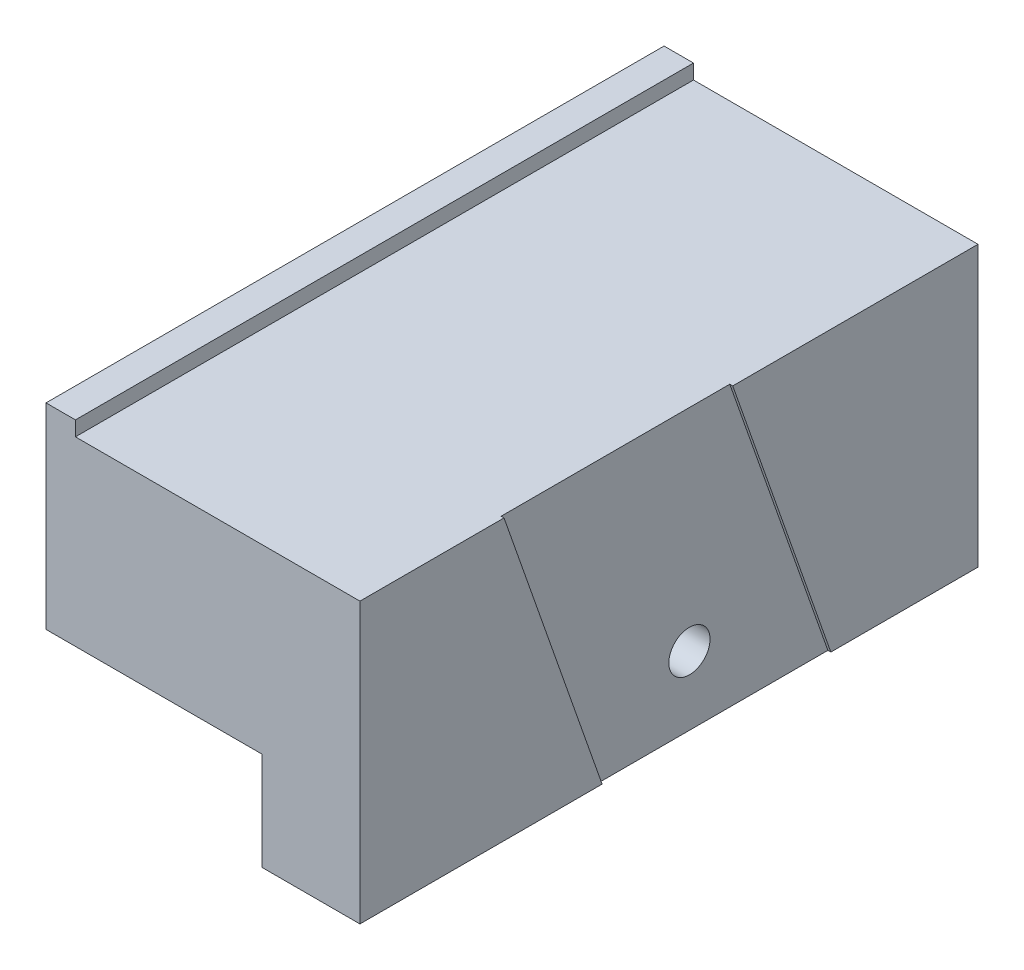
SolidWorks part; units mm, degrees
ref_plane "前视基准面" through (0, 0, 0) normal (0, 0, 1) x (1, 0, 0)
ref_plane "上视基准面" through (0, 0, 0) normal (0, 1, 0) x (1, 0, 0)
ref_plane "右视基准面" through (0, 0, 0) normal (1, 0, 0) x (0, 0, -1)
sketch "草图1" plane through (0, 0, 0) normal (0, 0, 1) x (1, 0, 0)
  line L0 (0, 0) -> (32, 0)
  line L1 (32, 0) -> (32, -30)
  line L2 (32, -30) -> (22, -30)
  line L3 (22, -30) -> (22, -20)
  line L4 (22, -20) -> (0, -20)
  line L5 (0, -20) -> (0, 0)
  dimension "D1" = 20
  dimension "D2" = 10
  dimension "D3" = 32
  dimension "D4" = 10
extrude "凸台-拉伸1" add sketch "草图1" along normal mid plane 63
sketch "草图2" plane through (0, 0, 0) normal (0, 1, 0) x (1, 0, 0)
  line L0 (32, -31.5) -> (0, -31.5) construction
  line L1 (32, 31.5) -> (3, 31.5)
  line L2 (32, 31.5) -> (32, -31.5)
  line L3 (32, -31.5) -> (3, -31.5)
  line L4 (3, 31.5) -> (3, -31.5)
  line L5 (0, -31.5) -> (0, 31.5) construction
  dimension "D1" = 3
extrude "切除-拉伸1" cut sketch "草图2" against normal blind 1.5
sketch "草图3" plane through (32, 0, 0) normal (1, 0, 0) x (0, 0, -1)
  line L0 (-16.815, -1.5) -> (-6.815, -30)
  line L1 (-31.5, -1.5) -> (31.5, -1.5) construction
  line L2 (-31.5, -30) -> (31.5, -30) construction
  line L3 (6.5, -1.5) -> (16.5, -30)
  line L4 (16.5, -30) -> (-6.815, -30)
  line L5 (-16.815, -1.5) -> (6.5, -1.5)
  line L6 (-5.1575, -1.5) -> (4.8425, -30) construction
  line L9 (31.5, -30) -> (31.5, -1.5) construction
  dimension "D1" = 22
  dimension "D2" = 15
  dimension "D3" = 25
extrude "切除-拉伸2" cut sketch "草图3" against normal blind 0.3
hole_wizard "M5 螺纹孔1" positions "3D草图1" profile "草图5" tap size "M5" standard "GB" end condition up to next
sketch3d "3D草图1"
  line L0 (31.7, -30, -4.8425) -> (31.7, -23, -2.3864)
  line L1 (31.7, -30, 6.815) -> (31.7, -30, -16.5) construction
  line L3 (31.7, -30, -16.5) -> (31.7, -1.5, -6.5) construction
  point P0 (31.7, -23, -2.3864)
  dimension "D1" = 7
sketch "草图5" plane through (31.7, -23, -2.3864) normal (0, 1, 0) x (0, 0, -1)
  line L0 (0, 0) -> (0, 9.7)
  line L1 (0, 9.7) -> (2.1, 9.7)
  line L2 (2.1, 9.7) -> (2.1, 0)
  line L5 (2.1, 0) -> (0, 0)
  line L11 (0, -6.35) -> (0, 107.95) construction
  dimension "通孔螺纹孔钻头直径" = 4.2
  dimension "通孔螺纹孔钻头深度" = 9.7
cosmetic thread "孔螺蚊线1" parameters "D2"=5
